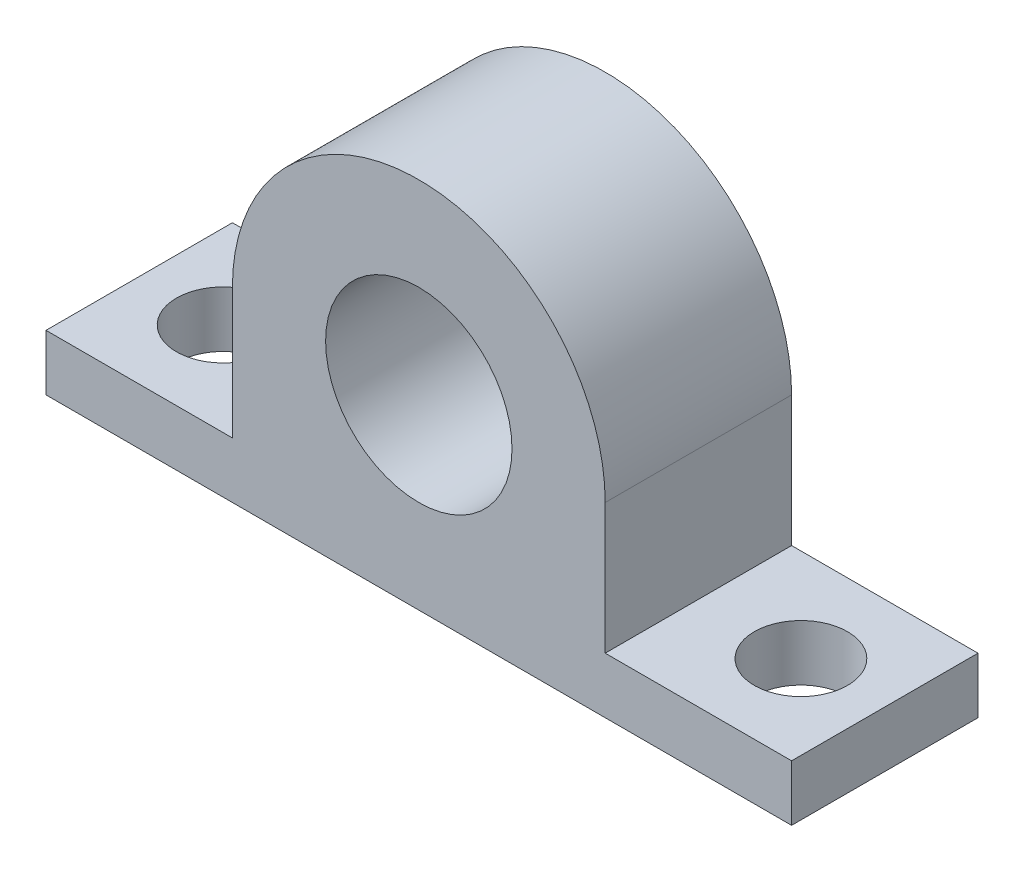
SolidWorks part; units mm, degrees
material "AISI 304"
ref_plane "Front Plane" through (0, 0, 0) normal (0, 0, 1) x (1, 0, 0)
ref_plane "Top Plane" through (0, 0, 0) normal (0, 1, 0) x (1, 0, 0)
ref_plane "Right Plane" through (0, 0, 0) normal (1, 0, 0) x (0, 0, -1)
other "Configuration Table"
sketch "Sketch1" plane through (0, 0, 0) normal (0, 0, 1) x (1, 0, 0)
  line L0 (-40, -20) -> (40, -20)
  line L1 (-40, -20) -> (-40, -14)
  line L2 (-40, -14) -> (40, -14)
  line L3 (40, -14) -> (40, -20)
  line L4 (0, 0) -> (0, -52.6012) construction
  line L5 (-20, 0) -> (-20, -28.31)
  line L6 (20, 0) -> (20, -30.8105)
  circle A0 centre (0, 0) radius 10
  circle A1 centre (0, 0) radius 20
  point P7 (0, -20)
  dimension "D1" = 20
  dimension "D2" = 40
  dimension "D3" = 80
  dimension "D4" = 6
extrude "Boss-Extrude1" add sketch "Sketch1" along normal mid plane 20
sketch "Sketch2" plane through (0, -14, 0) normal (0, 1, 0) x (1, 0, 0)
  circle A0 centre (0, 0) radius 31 construction
  circle A1 centre (31, 0) radius 5
  circle A2 centre (-31, 0) radius 5
  dimension "D1" = 62
  dimension "D2" = 10
  dimension "D3" = 10
extrude "Cut-Extrude1" cut sketch "Sketch2" against normal mid plane 20
